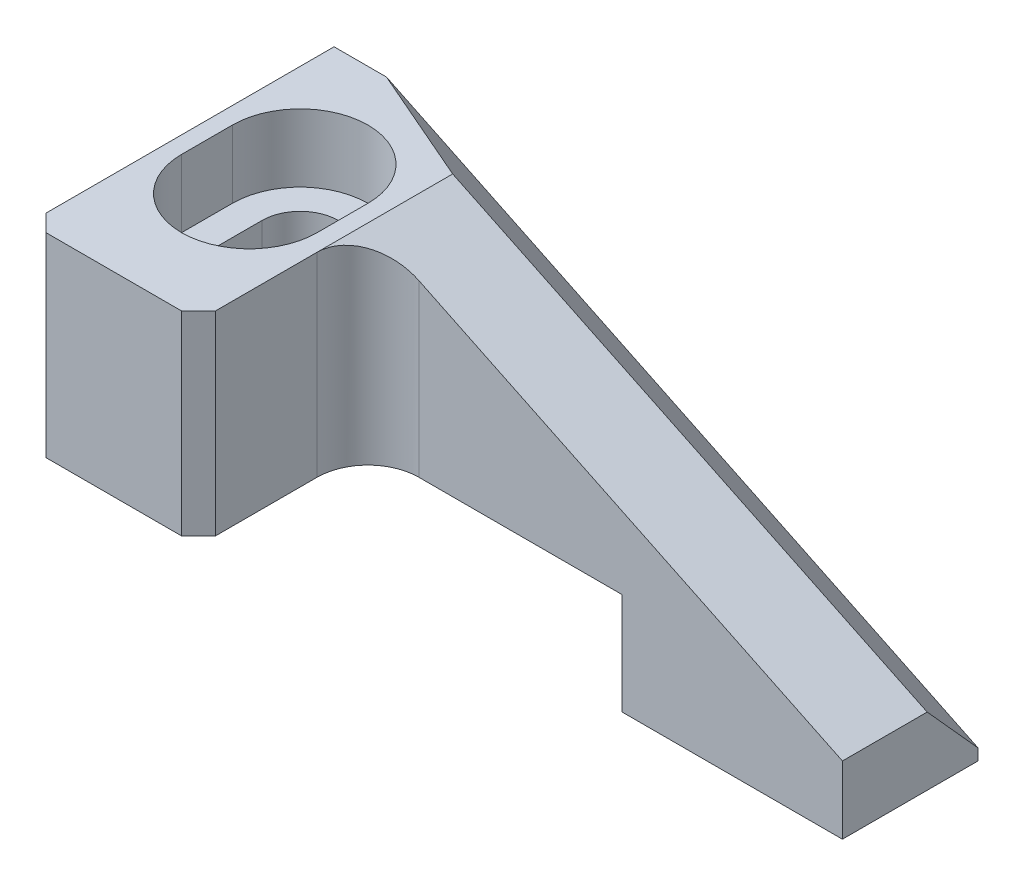
SolidWorks part; units mm, degrees
material "S45C"
ref_plane "Front Plane" through (0, 0, 0) normal (0, 0, 1) x (1, 0, 0)
ref_plane "Top Plane" through (0, 0, 0) normal (0, 1, 0) x (1, 0, 0)
ref_plane "Right Plane" through (0, 0, 0) normal (1, 0, 0) x (0, 0, -1)
sketch "Sketch1" plane through (0, 0, 0) normal (0, 0, 1) x (1, 0, 0)
  line L0 (0, 17.5) -> (0, 0)
  line L1 (0, 0) -> (38, 0)
  line L2 (38, 0) -> (38, 4)
  line L3 (38, 4) -> (10, 17.5)
  line L4 (10, 17.5) -> (0, 17.5)
  dimension "D1" = 10
  dimension "D2" = 38
  dimension "D3" = 4
  dimension "D4" = 17.5
extrude "Boss-Extrude1" add sketch "Sketch1" along normal blind 18
chamfer "Chamfer1" distance 3 distance2 3 1 edges at (24, 10.75, 0)
sketch "Sketch2" plane through (0, 17.5, 0) normal (0, 1, 0) x (1, 0, 0)
  line L0 (5, -10) -> (5, -7) construction
  line L1 (2.75, -10) -> (2.75, -7)
  line L2 (7.25, -10) -> (7.25, -7)
  line L3 (0, -18) -> (0, 0) construction
  line L4 (3.0923, 0) -> (0, 0) construction
  arc A0 (2.75, -10) -> (7.25, -10) centre (5, -10) ccw
  arc A1 (7.25, -7) -> (2.75, -7) centre (5, -7) ccw
  point P2 (5, -8.5)
  dimension "D1" = 3
  dimension "D3" = 2.25
  dimension "D4" = 7
  dimension "D2" = 5
extrude "Cut-Extrude1" cut sketch "Sketch2" against normal blind 20
sketch "Sketch4" plane through (0, 17.5, 0) normal (0, 1, 0) x (1, 0, 0)
  line L0 (5, -7) -> (5, -10) construction
  line L1 (9, -7) -> (9, -10)
  line L2 (1, -7) -> (1, -10)
  arc A0 (9, -7) -> (1, -7) centre (5, -7) ccw
  arc A1 (1, -10) -> (9, -10) centre (5, -10) ccw
  point P4 (5, -8.5)
  dimension "D1" = 4
extrude "Cut-Extrude3" cut sketch "Sketch4" against normal blind 4
sketch "Sketch3" plane through (0, 0, 18) normal (0, 0, 1) x (1, 0, 0)
  line L1 (0, 0) -> (25, 0)
  line L2 (0, 0) -> (0, 6)
  line L3 (0, 6) -> (25, 6)
  line L4 (25, 0) -> (25, 6)
  dimension "D1" = 6
  dimension "D2" = 25
extrude "Cut-Extrude2" cut sketch "Sketch3" against normal through all
sketch "Sketch5" plane through (0, 17.5, 0) normal (0, 1, 0) x (1, 0, 0)
  line L0 (38, -18) -> (38, -3) construction
  line L1 (10, -18) -> (38, -18)
  line L2 (10, -18) -> (10, -8)
  line L3 (10, -8) -> (38, -8)
  line L4 (38, -18) -> (38, -8)
  dimension "D1" = 10
extrude "Cut-Extrude4" cut sketch "Sketch5" against normal through all
fillet "Fillet1" radius 3 1 edges at (10, 11.75, 8)
chamfer "Chamfer2" distance 1 angle 45 2 edges at (10, 11.75, 18) (0, 11.75, 18)
